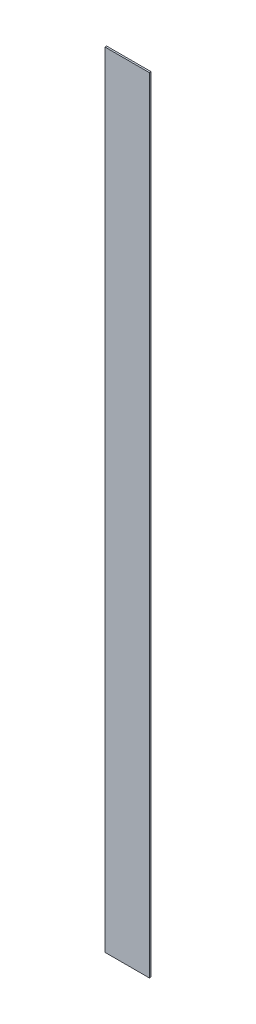
from build123d import *

# Parameters (mm, degrees)
SKETCH_1_W      = 131
SKETCH_1_H      = 2310
EXTRUDE_1_DEPTH = 5


with BuildPart() as part:
    # 草图1 → 凸台-拉伸1 (new body)
    with BuildSketch(Plane.XY):
        Rectangle(SKETCH_1_W, SKETCH_1_H)
    extrude(amount=EXTRUDE_1_DEPTH)


solid = part.part
